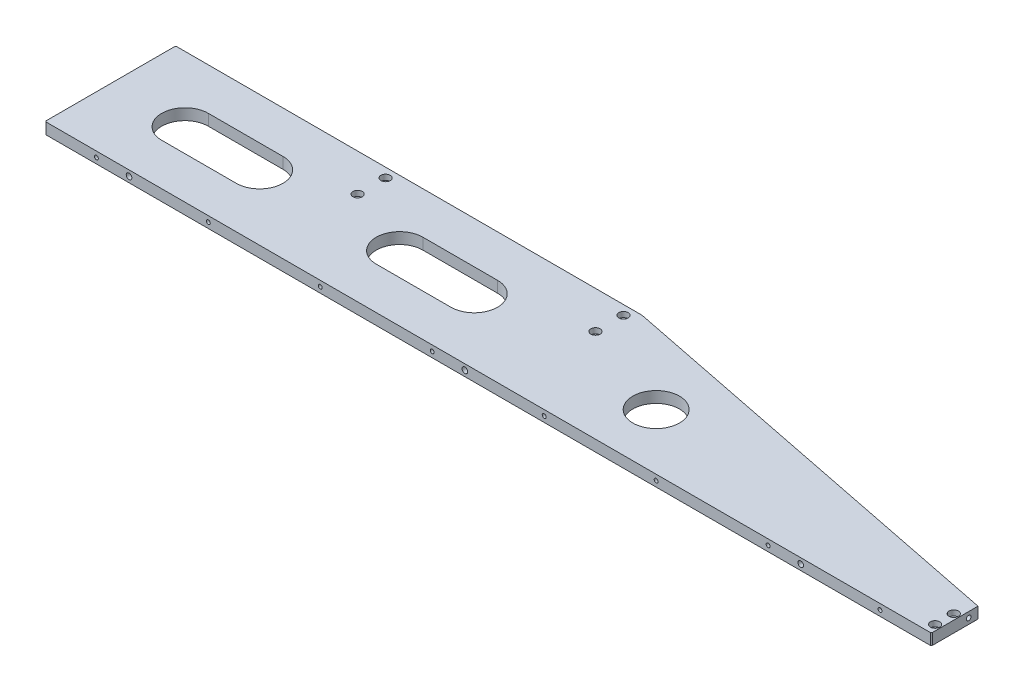
from build123d import *

# Parameters (mm, degrees)
BOSS_EXTRUDE2_DEPTH                              = 12
SKETCH9_R                                        = 25
CUT_EXTRUDE3_DEPTH                               = 12
M4_TAPPED_HOLE3_D                                = 3.3
M4_TAPPED_HOLE3_DEPTH                            = 11.5
M4_TAPPED_HOLE3_TIP                              = 0.991420021
M4_TAPPED_HOLE4_D                                = 3.3
M4_TAPPED_HOLE4_DEPTH                            = 11.5
M4_TAPPED_HOLE4_TIP                              = 0.991420021
M6_TAPPED_HOLE3_D                                = 5
M6_TAPPED_HOLE3_DEPTH                            = 17
M6_TAPPED_HOLE3_TIP                              = 1.502151548
M6_TAPPED_HOLE2_D                                = 5
M6_TAPPED_HOLE2_DEPTH                            = 23
M6_TAPPED_HOLE2_TIP                              = 1.502151548
F_6_0_6_DIAMETER_HOLE1_D                         = 6
F_6_0_6_DIAMETER_HOLE1_DEPTH                     = 15
F_6_0_6_DIAMETER_HOLE1_TIP                       = 1.802581857
M5_TAPPED_HOLE1_D                                = 4.2
M5_TAPPED_HOLE1_DEPTH                            = 12.4
M5_TAPPED_HOLE1_TIP                              = 1.2618073
F_6_0_6_DIAMETER_HOLE2_D                         = 6
F_6_0_6_DIAMETER_HOLE2_DEPTH                     = 15
F_6_0_6_DIAMETER_HOLE2_TIP                       = 1.802581857
HOLE_SIZE_PER_HEX_SOCKET_SCREW_TYPE1_D           = 5.5
HOLE_SIZE_PER_HEX_SOCKET_SCREW_TYPE1_CBORE_D     = 10
HOLE_SIZE_PER_HEX_SOCKET_SCREW_TYPE1_CBORE_DEPTH = 5.7
CHAMFER1_SIZE                                    = 1


with BuildPart() as part:
    # Sketch2 → Boss-Extrude2 (new body)
    with BuildSketch(Plane(origin=(0, 0, 0), x_dir=(-1, 0, 0), z_dir=(0, -1, 0))):
        Polygon((0, 0), (0, 140), (-500, 140), (-950, 50), (-950, 0), align=None)
    extrude(amount=-BOSS_EXTRUDE2_DEPTH)

    # Sketch9 → Cut-Extrude3 (cut)
    with BuildSketch(Plane.XZ):
        with Locations((595, -60)):
            Circle(SKETCH9_R)
        with BuildLine():
            Line((80, -45), (160, -45))
            ThreePointArc((160, -45), (185, -70), (160, -95))
            Line((160, -95), (80, -95))
            ThreePointArc((80, -95), (55, -70), (80, -45))
        make_face()
        with BuildLine():
            Line((310, -45), (390, -45))
            ThreePointArc((390, -45), (415, -70), (390, -95))
            Line((390, -95), (310, -95))
            ThreePointArc((310, -95), (285, -70), (310, -45))
        make_face()
    extrude(amount=-CUT_EXTRUDE3_DEPTH, mode=Mode.SUBTRACT)

    # M4 Tapped Hole3
    with Locations(Plane(origin=(0, 0, -140), x_dir=(-1, 0, 0), z_dir=(0, 0, -1))):
        with Locations((-50, 6), (-400, 6)):
            Hole(M4_TAPPED_HOLE3_D / 2, depth=M4_TAPPED_HOLE3_DEPTH)
            with Locations((0, 0, -(M4_TAPPED_HOLE3_DEPTH + M4_TAPPED_HOLE3_TIP / 2))):  # 118° drill point
                Cone(0, M4_TAPPED_HOLE3_D / 2, M4_TAPPED_HOLE3_TIP, mode=Mode.SUBTRACT)

    # M4 Tapped Hole4
    with Locations(Plane(origin=(46.153846154, 0, -230.769230769), x_dir=(-0.9805806756909201, 0, -0.19611613513818424), z_dir=(0.19611613513818424, 0, -0.9805806756909201))):
        with Locations((-871.745835149, 6), (-521.745835149, 6)):
            Hole(M4_TAPPED_HOLE4_D / 2, depth=M4_TAPPED_HOLE4_DEPTH)
            with Locations((0, 0, -(M4_TAPPED_HOLE4_DEPTH + M4_TAPPED_HOLE4_TIP / 2))):  # 118° drill point
                Cone(0, M4_TAPPED_HOLE4_D / 2, M4_TAPPED_HOLE4_TIP, mode=Mode.SUBTRACT)

    # M6 Tapped Hole3
    with Locations(Plane(origin=(950, 0, 0), x_dir=(0, 0, -1), z_dir=(1, 0, 0))):
        with Locations((40, 6), (40, 96)):
            Hole(M6_TAPPED_HOLE3_D / 2, depth=M6_TAPPED_HOLE3_DEPTH)
            with Locations((0, 0, -(M6_TAPPED_HOLE3_DEPTH + M6_TAPPED_HOLE3_TIP / 2))):  # 118° drill point
                Cone(0, M6_TAPPED_HOLE3_D / 2, M6_TAPPED_HOLE3_TIP, mode=Mode.SUBTRACT)

    # M6 Tapped Hole2
    with Locations(Plane.ZY):
        with Locations((-15, 6), (-70, 6), (-125, 6)):
            Hole(M6_TAPPED_HOLE2_D / 2, depth=M6_TAPPED_HOLE2_DEPTH)
            with Locations((0, 0, -(M6_TAPPED_HOLE2_DEPTH + M6_TAPPED_HOLE2_TIP / 2))):  # 118° drill point
                Cone(0, M6_TAPPED_HOLE2_D / 2, M6_TAPPED_HOLE2_TIP, mode=Mode.SUBTRACT)

    # Ø6.0 (6) Diameter Hole1
    with Locations(Plane.ZY):
        with Locations((-30, 6), (-110, 6)):
            Hole(F_6_0_6_DIAMETER_HOLE1_D / 2, depth=F_6_0_6_DIAMETER_HOLE1_DEPTH)
            with Locations((0, 0, -(F_6_0_6_DIAMETER_HOLE1_DEPTH + F_6_0_6_DIAMETER_HOLE1_TIP / 2))):  # 118° drill point
                Cone(0, F_6_0_6_DIAMETER_HOLE1_D / 2, F_6_0_6_DIAMETER_HOLE1_TIP, mode=Mode.SUBTRACT)

    # M5 Tapped Hole1
    with Locations(Plane.XY):
        with Locations((55, 6), (175, 6), (295, 6), (415, 6), (535, 6), (655, 6), (775, 6), (895, 6)):
            Hole(M5_TAPPED_HOLE1_D / 2, depth=M5_TAPPED_HOLE1_DEPTH)
            with Locations((0, 0, -(M5_TAPPED_HOLE1_DEPTH + M5_TAPPED_HOLE1_TIP / 2))):  # 118° drill point
                Cone(0, M5_TAPPED_HOLE1_D / 2, M5_TAPPED_HOLE1_TIP, mode=Mode.SUBTRACT)

    # Ø6.0 (6) Diameter Hole2
    with Locations(Plane.XY):
        with Locations((90, 6), (450, 6), (810, 6)):
            Hole(F_6_0_6_DIAMETER_HOLE2_D / 2, depth=F_6_0_6_DIAMETER_HOLE2_DEPTH)
            with Locations((0, 0, -(F_6_0_6_DIAMETER_HOLE2_DEPTH + F_6_0_6_DIAMETER_HOLE2_TIP / 2))):  # 118° drill point
                Cone(0, F_6_0_6_DIAMETER_HOLE2_D / 2, F_6_0_6_DIAMETER_HOLE2_TIP, mode=Mode.SUBTRACT)

    # Hole size per hex socket screw type1 (through all)
    with Locations(Plane(origin=(-526.958693224, 12, -55.479422486), x_dir=(-1, 0, 0), z_dir=(0, 1, 0))):
        with Locations((-761.958693224, -44.520577514), (-761.958693224, -74.520577514), (-1016.958693224, -44.520577514), (-1016.958693224, -74.520577514), (-1470.958693224, 45.479422486), (-1470.958693224, 25.479422486)):
            CounterBoreHole(HOLE_SIZE_PER_HEX_SOCKET_SCREW_TYPE1_D / 2, HOLE_SIZE_PER_HEX_SOCKET_SCREW_TYPE1_CBORE_D / 2, HOLE_SIZE_PER_HEX_SOCKET_SCREW_TYPE1_CBORE_DEPTH)

    # Chamfer1
    chamfer1_edges = [part.edges().sort_by_distance(p)[0] for p in [
        (950, 6, 0),
        (0, 6, -140),
        (0, 6, 0),
    ]]
    chamfer(chamfer1_edges, length=CHAMFER1_SIZE)


solid = part.part
